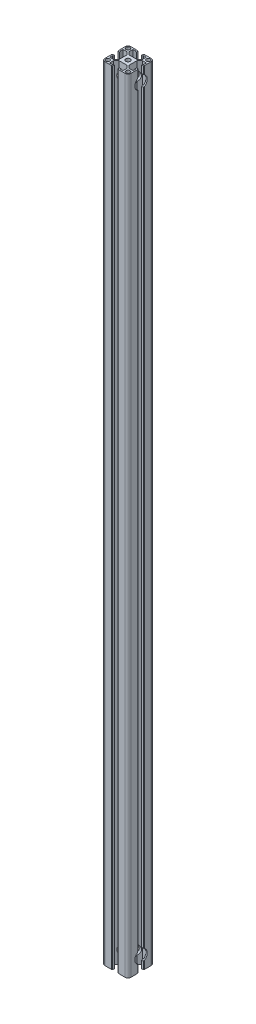
SolidWorks part; units mm, degrees
ref_plane "主视基准图" through (0, 0, 0) normal (0, 0, 1) x (1, 0, 0)
ref_plane "上视基准图" through (0, 0, 0) normal (0, 1, 0) x (1, 0, 0)
ref_plane "右视基准图" through (0, 0, 0) normal (1, 0, 0) x (0, 0, -1)
sketch "草图1" plane through (0, 0, 0) normal (0, 0, 1) x (1, 0, 0)
  line L0 (0, 0) -> (0, 1203)
  dimension "D1" = 1203
other "结构构件1"
ref_plane "基准面1" through (0, 0, 0) normal (0, 1, 0) x (-1, 0, 0)
sketch "Sketch16" plane through (0, 0, 0) normal (0, 1, 0) x (-1, 0, 0)
  line L0 (-5.1, 20) -> (-5.1, 19.5)
  line L1 (-5.1, 19.5) -> (-4.1, 19.5)
  line L2 (-4.1, 19.5) -> (-4.1, 17)
  line L3 (-6.1, 18) -> (-10.3, 18)
  line L4 (-15.5, -20) -> (-5.1, -20)
  line L5 (-20, -15.5) -> (-20, -5.1)
  line L6 (15.5, 20) -> (5.1, 20)
  line L7 (20, 15.5) -> (20, 5.1)
  line L8 (0, 14.8756) -> (0, 0) construction
  line L9 (0, 0) -> (14.1675, 0) construction
  line L10 (-10.3, 18) -> (-10.3, 12)
  line L11 (-10.3, 12) -> (-6, 7.7)
  line L12 (-6, 7.7) -> (6, 7.7)
  line L13 (10.3, 12) -> (6, 7.7)
  line L14 (10.3, 18) -> (10.3, 12)
  line L15 (6.1, 18) -> (10.3, 18)
  line L16 (4.1, 19.5) -> (4.1, 17)
  line L17 (5.1, 19.5) -> (4.1, 19.5)
  line L18 (5.1, 20) -> (5.1, 19.5)
  line L19 (-5.1, 20) -> (-15.5, 20)
  line L20 (20, 5.1) -> (19.5, 5.1)
  line L21 (0, 0) -> (-15.5563, 15.5563) construction
  line L22 (0, 0) -> (-15.5563, -15.5563) construction
  line L25 (19.5, 5.1) -> (19.5, 4.1)
  line L26 (19.5, 4.1) -> (17, 4.1)
  line L27 (17, 6.1) -> (17, 4.1)
  line L28 (18, 6.1) -> (17, 6.1)
  line L29 (18, 6.1) -> (18, 10.3)
  line L30 (18, 10.3) -> (12, 10.3)
  line L31 (12, 10.3) -> (7.7, 6)
  line L32 (7.7, 6) -> (7.7, -6)
  line L33 (12, -10.3) -> (7.7, -6)
  line L34 (18, -10.3) -> (12, -10.3)
  line L35 (18, -6.1) -> (18, -10.3)
  line L36 (18, -6.1) -> (17, -6.1)
  line L37 (17, -4.1) -> (17, -6.1)
  line L38 (19.5, -4.1) -> (17, -4.1)
  line L39 (19.5, -5.1) -> (19.5, -4.1)
  line L40 (20, -5.1) -> (19.5, -5.1)
  line L41 (5.1, -20) -> (5.1, -19.5)
  line L42 (5.1, -19.5) -> (4.1, -19.5)
  line L43 (4.1, -19.5) -> (4.1, -17)
  line L44 (6.1, -17) -> (4.1, -17)
  line L45 (6.1, -18) -> (6.1, -17)
  line L46 (6.1, -18) -> (10.3, -18)
  line L47 (10.3, -18) -> (10.3, -12)
  line L48 (10.3, -12) -> (6, -7.7)
  line L49 (6, -7.7) -> (-6, -7.7)
  line L50 (-10.3, -12) -> (-6, -7.7)
  line L51 (-10.3, -18) -> (-10.3, -12)
  line L52 (-6.1, -18) -> (-10.3, -18)
  line L53 (-6.1, -18) -> (-6.1, -17)
  line L54 (-4.1, -17) -> (-6.1, -17)
  line L55 (-4.1, -19.5) -> (-4.1, -17)
  line L56 (-5.1, -19.5) -> (-4.1, -19.5)
  line L57 (-5.1, -20) -> (-5.1, -19.5)
  line L58 (-20, -5.1) -> (-19.5, -5.1)
  line L59 (5.1, -20) -> (15.5, -20)
  line L60 (-20, 5.1) -> (-20, 15.5)
  line L61 (-19.5, -5.1) -> (-19.5, -4.1)
  line L62 (-6.1, 18) -> (-6.1, 17)
  line L63 (-6.1, 17) -> (-4.1, 17)
  line L64 (6.1, 18) -> (6.1, 17)
  line L65 (4.1, 17) -> (6.1, 17)
  line L66 (-19.5, -4.1) -> (-17, -4.1)
  line L71 (-17, -6.1) -> (-17, -4.1)
  line L72 (-18, -6.1) -> (-17, -6.1)
  line L73 (-18, -6.1) -> (-18, -10.3)
  line L74 (-18, -10.3) -> (-12, -10.3)
  line L75 (-12, -10.3) -> (-7.7, -6)
  line L76 (-7.7, -6) -> (-7.7, 6)
  line L77 (-12, 10.3) -> (-7.7, 6)
  line L78 (-18, 10.3) -> (-12, 10.3)
  line L79 (-18, 6.1) -> (-18, 10.3)
  line L80 (-18, 6.1) -> (-17, 6.1)
  line L81 (-17, 4.1) -> (-17, 6.1)
  line L82 (-19.5, 4.1) -> (-17, 4.1)
  line L83 (-19.5, 5.1) -> (-19.5, 4.1)
  line L84 (-20, 5.1) -> (-19.5, 5.1)
  line L85 (20, -5.1) -> (20, -15.5)
  circle A0 centre (0, 0) radius 3.4
  arc A1 (-20, 15.5) -> (-15.5, 20) centre (-15.5, 15.5) cw
  arc A2 (20, 15.5) -> (15.5, 20) centre (15.5, 15.5) ccw
  arc A3 (-15.5, -20) -> (-20, -15.5) centre (-15.5, -15.5) cw
  arc A4 (15.5, -20) -> (20, -15.5) centre (15.5, -15.5) ccw
  circle A5 centre (-15.5563, 15.5563) radius 3
  circle A6 centre (15.5563, 15.5563) radius 3
  circle A7 centre (15.5563, -15.5563) radius 3
  circle A8 centre (-15.5563, -15.5563) radius 3
  point P2 (0, 10)
  point P3 (0, 0)
  point P4 (0, 0)
  point P5 (-20, -20)
  point P6 (20, -20)
  point P7 (20, 20)
  point P8 (-20, 20)
  point P36 (-20, 20)
  point P39 (20, 20)
  dimension "D1" = 20.6
  dimension "D2" = 40
  dimension "D3" = 8.2
  dimension "D4" = 10.2
  dimension "D5" = 12.3
  dimension "D6" = 6.8
  dimension "D7" = 4.5
  dimension "D8" = 45
  dimension "D12" = 6
  dimension "D13" = 22
  dimension "D9" = 0.5
  dimension "D10" = 2
  dimension "D11" = 12
  dimension "D16" = 3
  dimension "D17" = 2
sketch "草图2" plane through (-20, 0, 0) normal (-1, 0, 0) x (0, 0, 1)
  line L0 (-7.7, 0) -> (-12, 0) construction
  line L1 (-15.5, 1203) -> (-5.1, 1203) construction
  circle A0 centre (0, 1183) radius 9.5
  circle A1 centre (0, 20) radius 9.5
  point P4 (-9.85, 0)
  dimension "D1" = 19
  dimension "D2" = 19
  dimension "D3" = 20
  dimension "D4" = 20
extrude "切除-拉伸1" cut sketch "草图2" against normal through all
